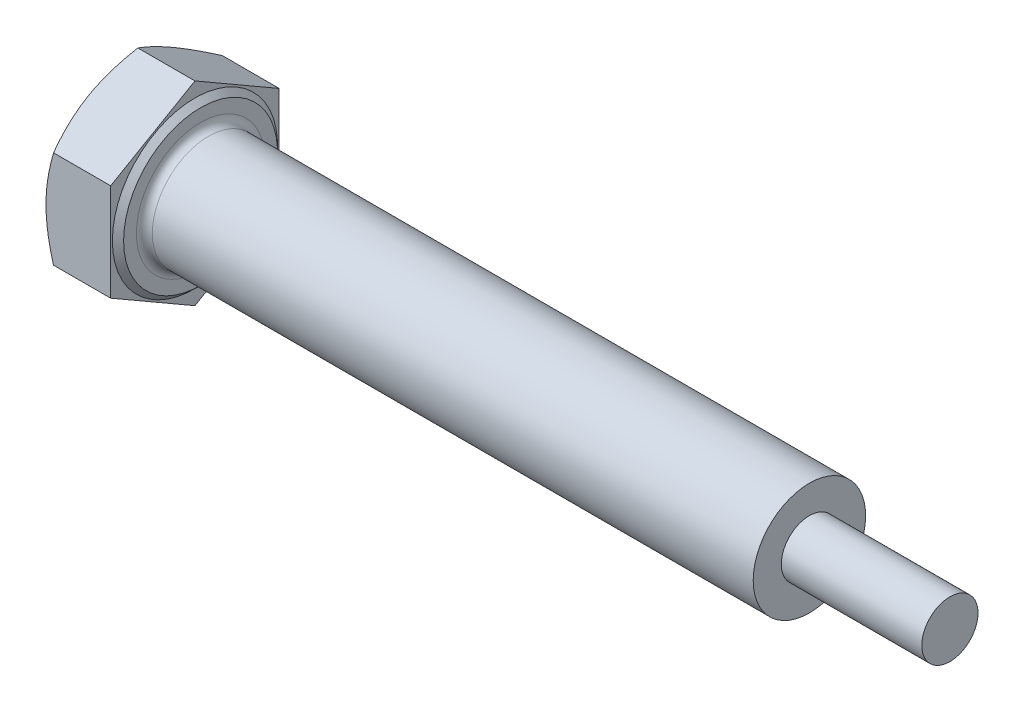
SolidWorks part; units mm, degrees
material "钢"
ref_plane "Front Plane" through (0, 0, 0) normal (0, 0, 1) x (1, 0, 0)
ref_plane "Top Plane" through (0, 0, 0) normal (0, 1, 0) x (1, 0, 0)
ref_plane "Right Plane" through (0, 0, 0) normal (1, 0, 0) x (0, 0, -1)
sketch "Sketch1" plane through (0, 0, 0) normal (0, 0, 1) x (1, 0, 0)
  line L0 (0, 0) -> (87.5, 0) construction
  line L1 (0, 0) -> (0, 10.015)
  line L2 (0, 10.015) -> (7.5, 10.015)
  line L3 (7.5, 10.015) -> (7.5, 0)
  line L4 (7.5, 6) -> (87.5, 6)
  line L5 (87.5, 6) -> (87.5, 0)
  line L6 (0, 9) -> (0.586, 10.015)
  line L7 (84, 6) -> (84, 0)
  line L8 (12.8, 6) -> (12.8, 0)
  line L9 (7.5, 5.4317) -> (87.5, 5.4317)
  line L10 (87.5, 5.0528) -> (7.5, 5.0528)
  line L11 (6.9, 8.815) -> (7.5, 8.215)
  line L12 (6.9, 10.015) -> (6.9, 0)
  line L13 (7.4, 8.315) -> (7.4, 0) construction
  arc A0 (7.5, 6.85) -> (8.35, 6) centre (8.35, 6.85) ccw
  point P12 (85.75, 0)
  point P13 (2.38, 10.015)
  point P14 (7.5, 6.85)
  point P24 (7.5, 8.315)
  dimension "D1" = 0.1
  dimension "r" = 0.85
  dimension "k" = 7.5
  dimension "D2" = 45
  dimension "β" = 30
  dimension "e" = 20.03
  dimension "s" = 18
  dimension "d" = 12
  dimension "l" = 80
  dimension "D52" = 3.5
  dimension "P" = 1.75
  dimension "kw" = 5.12
  dimension "da" = 13.7
  dimension "a" = 5.3
  dimension "ds" = 10.8634
  dimension "D61" = 10.1056
  dimension "dw" = 16.63
  dimension "c" = 0.6
sketch "Sketch2" plane through (0, 0, 0) normal (1, 0, 0) x (0, 0, -1)
  line L1 (0, 10.3923) -> (-9, 5.1962)
  line L2 (-9, 5.1962) -> (-9, -5.1962)
  line L3 (-9, -5.1962) -> (0, -10.3923)
  line L4 (0, -10.3923) -> (9, -5.1962)
  line L5 (9, -5.1962) -> (9, 5.1962)
  line L6 (9, 5.1962) -> (0, 10.3923)
  circle A0 centre (0, 0) radius 9 construction
sketch "Sketch3" plane through (0, 0, 0) normal (1, 0, 0) x (0, 0, -1)
  line L0 (9, 5.1962) -> (0, 10.3923) construction
  line L1 (0, 10.3923) -> (-9, 5.1962) construction
  line L2 (-9, 5.1962) -> (-9, -5.1962) construction
  line L3 (9, -5.1962) -> (9, 5.1962) construction
  line L4 (0, -10.3923) -> (9, -5.1962) construction
  line L5 (-9, -5.1962) -> (0, -10.3923) construction
  line L6 (9, 5.1962) -> (0, 10.3923)
  line L7 (0, 10.3923) -> (-9, 5.1962)
  line L8 (-9, 5.1962) -> (-9, -5.1962)
  line L9 (9, -5.1962) -> (9, 5.1962)
  line L10 (0, -10.3923) -> (9, -5.1962)
  line L11 (-9, -5.1962) -> (0, -10.3923)
extrude "Boss-Extrude1" add sketch "Sketch3" along normal up to vertex (7.5 mm away) up to point (7.5, 10.015, 0)
sketch "Sketch4" plane through (0, 0, 0) normal (-1, 0, 0) x (0, 0, 1)
  circle A0 centre (0, 0) radius 9 construction
  circle A1 centre (0, 0) radius 9
  circle A2 centre (0, 0) radius 20.03
  dimension "D1" = 40.06
extrude "Cut-Extrude1" cut sketch "Sketch4" against normal blind 0.9375 draft 60
sketch "Sketch5" plane through (0, 0, 0) normal (0, 0, 1) x (1, 0, 0)
  line L0 (7.5, 6) -> (87.5, 6) construction
  line L1 (87.5, 6) -> (87.5, 0) construction
  line L2 (0, 0) -> (87.5, 0) construction
  line L3 (8.35, 6) -> (87.5, 6)
  line L4 (87.5, 6) -> (87.5, 0)
  line L5 (7.5, 0) -> (87.5, 0)
  line L6 (7.5, 6.85) -> (7.5, 0)
  arc A0 (7.5, 6.85) -> (8.35, 6) centre (8.35, 6.85) ccw construction
  arc A1 (7.5, 6.85) -> (8.35, 6) centre (8.35, 6.85) ccw
revolve "Revolve1" add sketch "Sketch5" angle 360 about L5
cosmetic thread "Cosmetic Thread2" parameters "D1"=59.7, "D2"=10.1056
chamfer "Chamfer2" distance 0.6667 angle 45 1 edges at (87.5, 0, 6)
sketch "Sketch7" plane through (0, 0, 0) normal (0, 0, 1) x (1, 0, 0)
  line L0 (7.5, 8.215) -> (6.9, 8.815)
  line L1 (6.9, 8.815) -> (6.9, 20.03)
  line L2 (6.9, 20.03) -> (7.5, 20.03)
  line L3 (7.5, 20.03) -> (7.5, 8.215)
  line L4 (0, 0) -> (87.5, 0) construction
  line L5 (0, 0) -> (87.5, 0) construction
  dimension "D1" = 40.06
revolve "Cut-Revolve1" cut sketch "Sketch7" angle 360 mid plane about L5
sketch "Sketch6" [suppressed] plane through (0, 0, 0) normal (0, 0, 1) x (1, 0, 0)
  line L0 (9.3, 0) -> (9.3, 4) construction
  line L1 (9.3, 4) -> (75.3, 4)
  line L2 (75.3, 4) -> (75.3, 0)
  line L3 (9.3, 4) -> (5.9719, 3.5984)
  line L5 (5.3, 3.5941) -> (75.3, 3.5941) construction
  line L6 (5.3, 7.19) -> (5.3, 0) construction
  line L7 (5.3, 4.1941) -> (5.3, 0)
  line L8 (5.3, 0) -> (75.3, 0)
  arc A0 (5.9719, 3.5984) -> (5.3, 4.1941) centre (5.9, 4.1941) cw
  arc A1 (5.3, 4.6) -> (5.9, 4) centre (5.9, 4.6) ccw construction
revolve "Revolve2" add sketch "Sketch6" angle 360 about L8
cosmetic thread "Cosmetic Thread1" [suppressed] parameters "D1"=74.7, "D2"=10.1056
chamfer "Chamfer1" [suppressed] distance 0.6667 angle 45
sketch "Sketch8" [suppressed] plane through (0, 0, 0) normal (0, 0, 1) x (1, 0, 0)
  line L0 (5.3, 5.715) -> (4.7, 6.315)
  line L1 (4.7, 6.315) -> (4.7, 14.38)
  line L2 (4.7, 14.38) -> (5.3, 14.38)
  line L3 (5.3, 14.38) -> (5.3, 5.715)
  line L4 (0, 0) -> (75.3, 0) construction
  line L5 (0, 0) -> (75.3, 0) construction
  dimension "D1" = 40.06
revolve "Cut-Revolve2" [suppressed] cut sketch "Sketch8" angle 360 mid plane about L5
sketch "Sketch9" plane through (87.5, 0, 0) normal (1, 0, 0) x (0, 0, -1)
  circle A0 centre (0, 0) radius 3
  circle A1 centre (0, 0) radius 8.815
  dimension "D1" = 6
extrude "Cut-Extrude2" cut sketch "Sketch9" against normal blind 15
